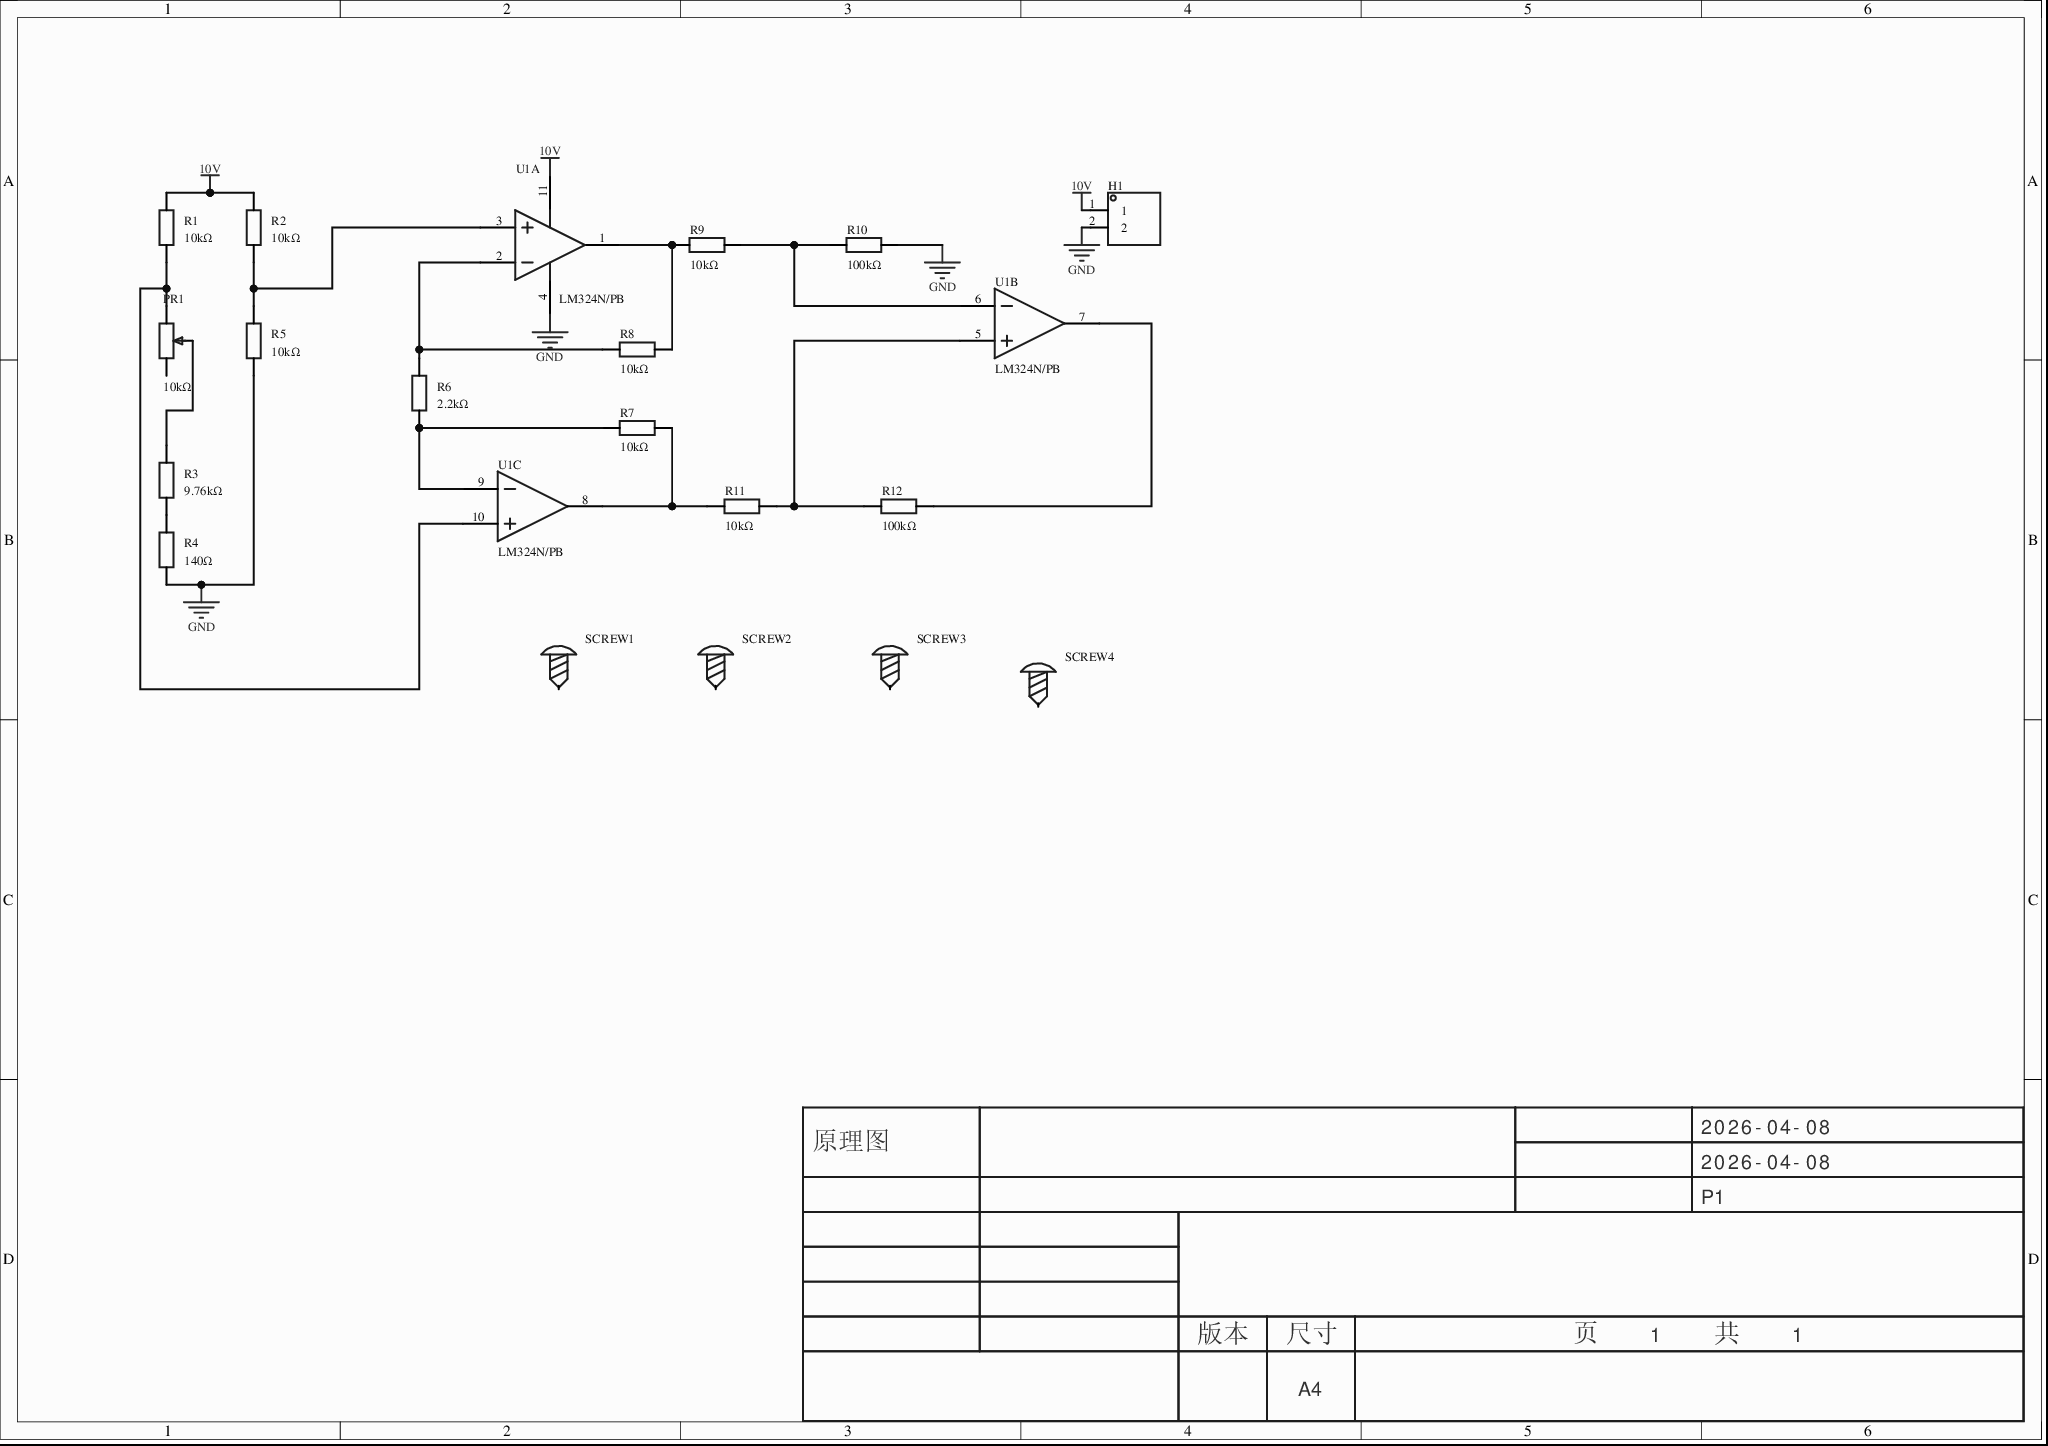
[diagram p0: MISC51917-3.schdoc]
# Altium project MISC51917-2.PrjPcb
1 sheet, 19 parts. Net scope: global (net labels, ports and power ports of the same name join across sheets).
Board file: MISC51917.pcbdoc

## Sheet MISC51917-3.schdoc
size 297 x 209 mm; Version: V1.0; @Project Name: MISC51917; @Update Date: 2026-04-08; @Create Date: 2026-04-08; @Board Name: MISC51917; @Create Time: 23:10:46; @Page Count: 1; @Page No: 1; @Schematic Name: MISC51917; @Update Time: 23:10:46; Size: A4

### Parts
H1  (no value)  [HDR-TH_2P-P2.54-V-M-1]
PR1  10kΩ  [R_3296]
R1  10kΩ  [Res_1/8W]
R2  10kΩ  [Res_1/8W]
R3  9.76kΩ  [Res_1/8W]
R4  140Ω  [Res_1/8W]
R5  10kΩ  [Res_1/8W]
R6  2.2kΩ  [Res_1/8W]
R7  10kΩ  [Res_1/8W]
R8  10kΩ  [Res_1/8W]
R9  10kΩ  [Res_1/8W]
R10  100kΩ  [Res_1/8W]
R11  10kΩ  [Res_1/8W]
R12  100kΩ  [Res_1/8W]
SCREW1  (no value)  [M2螺丝]
SCREW2  (no value)  [M2螺丝]
SCREW3  (no value)  [M2螺丝]
SCREW4  (no value)  [M2螺丝]
U1  LM324N/PB  [PDIP-14_L19.2-W6.6-P2.54-LS7.6-BL]  (parts A,B,C of 4)

### Nets
10V: H1.1 R1.2 R2.2 U1.11(GND)
GND: H1.2 R4.1 R5.1 R10.1 U1.4(V+)
NetPR1_2: PR1.2 R3.2
NetPR1_3: PR1.3 R1.1 U1.10(INC+)
NetR2_1: R2.1 R5.2 U1.3(INA+)
NetR3_1: R3.1 R4.2
NetR6_1: R6.1 R7.2 U1.9(INC-)
NetR6_2: R6.2 R8.2 U1.2(INA-)
NetR7_1: R7.1 R11.2 U1.8(OUTC)
NetR8_1: R8.1 R9.2 U1.1(OUTA)
NetR9_1: R9.1 R10.2 U1.6(INB-)
NetR11_1: R11.1 R12.2 U1.5(INB+)
NetR12_1: R12.1 U1.7(OUTB)

Not connected (* = marked no-connect by the designer): PR1 1; SCREW1 1; SCREW2 1; SCREW3 1; SCREW4 1

### Notes on the sheet
- 2026-04-08
- 原理图
- P1
- 版本
- 尺寸
- A4
- 页    1    共    1

### Library data of the parts
H1 = HDR-M_2.54_1x2P: Symbol: 210S-1*2P L=11.6MMGold-plated black; ConvertToPcb: yes; ModelId: 79b2e9f2d70a4d68a1b7098f27c6d4c50819f05c4eef4c71ace90d822a990e87; ModelName: HDR-M-2.54_1x2; ModelTransform: 200,100,0,0,0,0,0,0,-118.11; Device: HDR-M_2.54_1x2P; AddInBom: yes; SupplierPart: C124375; Supplier Footprint: 插件; FootprintName: HDR-TH_2P-P2.54-V-M-1
PR1 = R_3296: ConvertToPcb: yes; ModelId: b182808559bb43bda9e7de64b64134cb0819f05c4eef4c71ace90d822a990e87; ModelName: 3296W; ModelTransform: 373.98,188.96,590.49,180,0,0,0,0,-140; Symbol: R_3296; Device: R_3296; AddInBom: yes; Supplier Footprint: 直插; FootprintName: R_3296; Value: 10kΩ
R1-R12 = Res_AXIAL-1/8W: Symbol: 电阻; ConvertToPcb: yes; ModelId: b2b5ae7ae4c642178fe0039925c86a3f0819f05c4eef4c71ace90d822a990e87; ModelName: RES-TH_BD1.8-L3.2-P7.20-D0.4; ModelTransform: 282.86,66.88,253.09,0,0,0,0,0,-191; Device: Res_AXIAL-1/8W; AddInBom: yes; Supplier Footprint: 轴向引线; FootprintName: Res_1/8W
  R1 R2 R5 R7-R9 R11: Value: 10kΩ
  R3: Value: 9.76kΩ
  R4: Value: 140Ω
  R6: Value: 2.2kΩ
  R10 R12: Value: 100kΩ
SCREW1-SCREW4 = M2螺丝: Symbol: 螺丝孔; ConvertToPcb: yes; Device: M2螺丝; AddInBom: yes; Supplier Footprint: 插件; FootprintName: M2螺丝
U1 = LM324N/PB: 放大器数:4;轨到轨:-;增益带宽积(GBW):-;输入失调电压(Vos):2mV;压摆率(SR):-;输入偏置电流(Ib):45nA;; Manufacturer: TI(德州仪器); Relevance: []; AddInBom: yes; ModelId: 08aeb3774ab0450ba412f07c9830bd710819f05c4eef4c71ace90d822a990e87; ModelTransform: 755.904,309.842,0,0,0,0,0,0,-129.921; Number of Channels: 4; Maximum Power Supply Range (Vdd-Vss): 32V; Vos - Input Offset Voltage: 2mV; Input Offset Voltage Drift(Vos TC): 7uV/℃; Ib - Input Bias Current: 45nA; Input Offset Current(Ios): 5nA; Common Mode Rejection Ratio(CMRR): 65dB; Quiescent Current: 700uA; Output Current: 40mA; Symbol: LM324N/PB; Device: LM324N/PB; LCSC Part Name: LM324N/PB; SupplierPart: C4366406; ManufacturerPart: LM324N/PB; Supplier Footprint: PDIP-14; JLCPCB Part Class: Extended Part; Datasheet: https://item.szlcsc.com/datasheet/LM324N%252FPB/4937320.html; Supplier: LCSC; ConvertToPcb: yes; FootprintName: PDIP-14_L19.2-W6.6-P2.54-LS7.6-BL; ModelName: PDIP-14_L19.2-W6.6-P2.54-LS7.6-BL; Rail to Rail: -; Gain Bandwidth Product: -; Slew Rate: -; Input Voltage Noise Density: -; Input offset current drift(Ios TC): -; Operating Temperature: 0℃~+70℃; Single supply: -; Dual Supply: -; Features: -